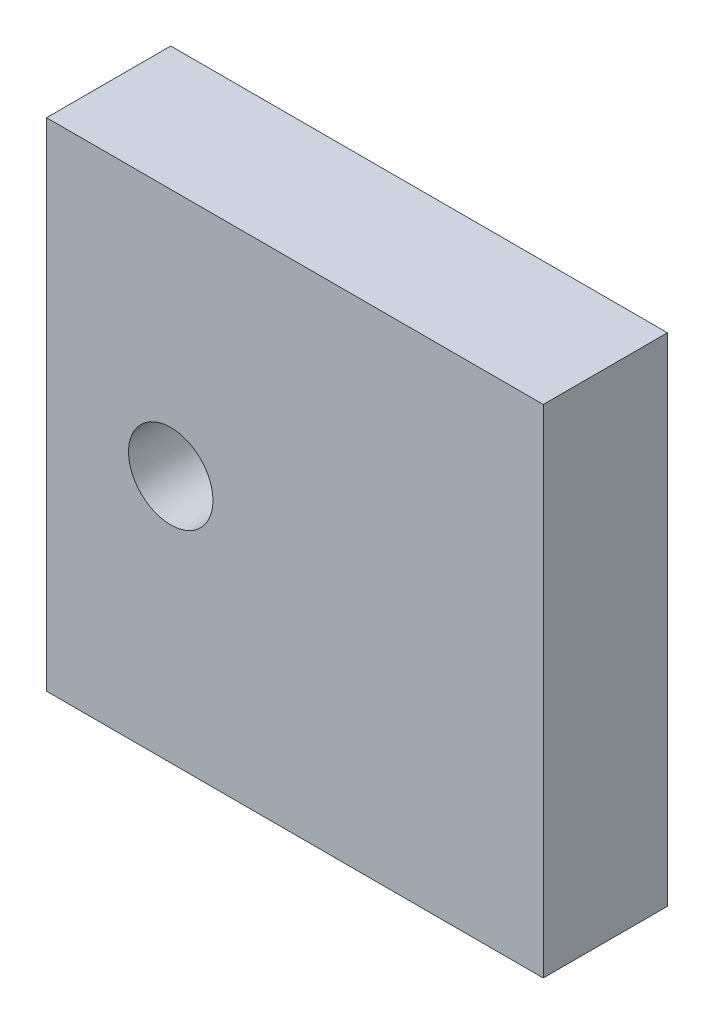
SolidWorks part; units mm, degrees
ref_plane "前视基准面" through (0, 0, 0) normal (0, 0, 1) x (1, 0, 0)
ref_plane "上视基准面" through (0, 0, 0) normal (0, 1, 0) x (1, 0, 0)
ref_plane "右视基准面" through (0, 0, 0) normal (1, 0, 0) x (0, 0, -1)
sketch "草图1" plane through (0, 0, 0) normal (0, 0, 1) x (1, 0, 0)
  line L1 (-20, -20) -> (20, -20)
  line L2 (-20, -20) -> (-20, 20)
  line L3 (-20, 20) -> (20, 20)
  line L4 (20, -20) -> (20, 20)
  line L5 (-20, -20) -> (20, 20) construction
  line L6 (-20, 20) -> (20, -20) construction
  point P0 (0, 0)
  dimension "D1" = 40
  dimension "D2" = 40
extrude "凸台-拉伸1" add sketch "草图1" along normal mid plane 10
hole_wizard "M8 螺纹孔1" positions "草图2" profile "草图3" tap size "M8" standard "GB" end condition through all
sketch "草图2" plane through (0, 0, 5) normal (0, 0, 1) x (1, 0, 0)
  line L0 (-20, 20) -> (-20, -20) construction
  line L1 (-20, -20) -> (20, -20) construction
  point P0 (-10, 0)
  dimension "D1" = 10
  dimension "D2" = 20
sketch "草图3" plane through (-10, 0, 5) normal (1, 0, 0) x (0, -1, 0)
  line L0 (0, 0) -> (0, 10)
  line L1 (0, 10) -> (3.4, 10)
  line L2 (3.4, 10) -> (3.4, 0)
  line L5 (3.4, 0) -> (0, 0)
  line L11 (0, -6.35) -> (0, 107.95) construction
  dimension "通孔螺纹孔钻头直径" = 6.8
  dimension "通孔螺纹孔钻头深度" = 10
cosmetic thread "孔螺蚊线1" parameters "D2"=8
